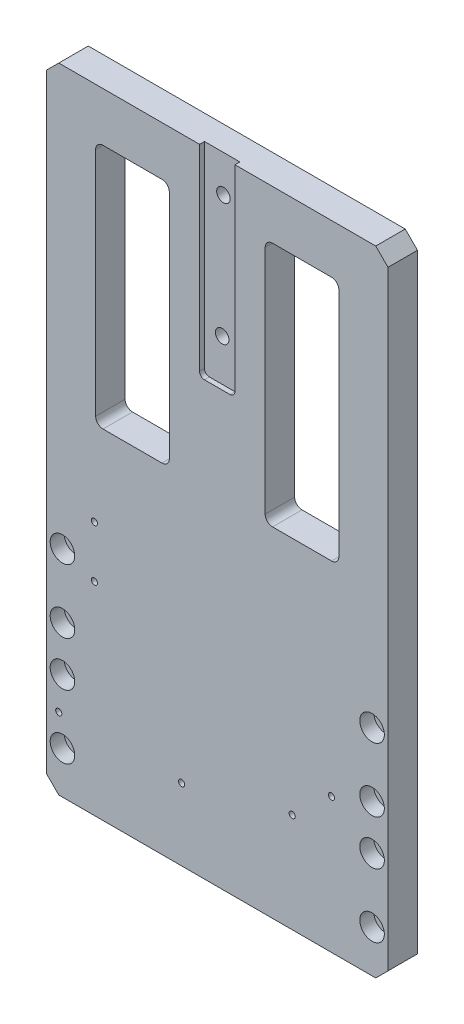
from build123d import *

# Parameters (mm, degrees)
SKETCH1_W                                            = 139
SKETCH1_H                                            = 258
BOSS_EXTRUDE1_DEPTH                                  = 12
CHAMFER1_SIZE                                        = 5
SKETCH2_W                                            = 30
SKETCH2_H                                            = 100
CUT_EXTRUDE1_DEPTH                                   = 237.506741929
SKETCH3_W                                            = 14.4
SKETCH3_H                                            = 82
CUT_EXTRUDE2_DEPTH                                   = 2
FILLET1_R                                            = 2
M3_TAPPED_HOLE1_D                                    = 2.5
M3_TAPPED_HOLE2_D                                    = 2.5
CBORE_FOR_M5_HEXAGON_SOCKET_HEAD_CAP_SCR_D           = 5.5
CBORE_FOR_M5_HEXAGON_SOCKET_HEAD_CAP_SCR_CBORE_D     = 10
CBORE_FOR_M5_HEXAGON_SOCKET_HEAD_CAP_SCR_CBORE_DEPTH = 5.7
FILLET2_R                                            = 3
CBORE_FOR_M5_HEXAGON_SOCKET_HEAD_CAP_2_D             = 5.5
CBORE_FOR_M5_HEXAGON_SOCKET_HEAD_CAP_2_DEPTH         = 11.5
CBORE_FOR_M5_HEXAGON_SOCKET_HEAD_CAP_2_CBORE_D       = 10
CBORE_FOR_M5_HEXAGON_SOCKET_HEAD_CAP_2_CBORE_DEPTH   = 5.7
CBORE_FOR_M5_HEXAGON_SOCKET_HEAD_CAP_2_TIP           = 1.652366702


with BuildPart() as part:
    # Sketch1 → Boss-Extrude1 (new body)
    with BuildSketch(Plane.XY):
        with Locations((50, 74.74294829)):
            Rectangle(SKETCH1_W, SKETCH1_H)
    extrude(amount=BOSS_EXTRUDE1_DEPTH)

    # Chamfer1
    chamfer1_edges = [part.edges().sort_by_distance(p)[0] for p in [
        (119.5, -54.25705171, 6),
        (-19.5, -54.25705171, 6),
        (-19.5, 203.74294829, 6),
        (119.5, 203.74294829, 6),
    ]]
    chamfer(chamfer1_edges, length=CHAMFER1_SIZE)

    # Sketch2 → Cut-Extrude1 (cut, through all)
    with BuildSketch(Plane.XY.offset(12)):
        with Locations((84.5, 133.74294829)):
            Rectangle(SKETCH2_W, SKETCH2_H)
        with Locations((15.5, 133.74294829)):
            Rectangle(SKETCH2_W, SKETCH2_H)
    extrude(amount=-CUT_EXTRUDE1_DEPTH, mode=Mode.SUBTRACT)

    # Sketch3 → Cut-Extrude2 (cut)
    with BuildSketch(Plane.XY.offset(12)):
        with Locations((50, 162.74294829)):
            Rectangle(SKETCH3_W, SKETCH3_H)
    extrude(amount=-CUT_EXTRUDE2_DEPTH, mode=Mode.SUBTRACT)

    # Fillet1
    fillet1_edges = [part.edges().sort_by_distance(p)[0] for p in [
        (57.2, 121.74294829, 11),
        (42.8, 121.74294829, 11),
    ]]
    fillet(fillet1_edges, radius=FILLET1_R)

    # M3 Tapped Hole1 (through all)
    with Locations(Plane.XY.offset(12)):
        with Locations((-14.5, -25.018399206), (35.5, -25.018399206), (96.5, 0.74294829), (80.5, -13.75705171)):
            Hole(M3_TAPPED_HOLE1_D / 2)

    # M3 Tapped Hole2 (through all)
    with Locations(Plane.XY.offset(12)):
        with Locations((0, 49.24294829), (0, 28.24294829)):
            Hole(M3_TAPPED_HOLE2_D / 2)

    # CBORE for M5 Hexagon socket head cap scr (through all)
    with Locations(Plane(origin=(0, 0, 0), x_dir=(-1, 0, 0), z_dir=(0, 0, -1))):
        with Locations((-50.5, 188.74294829), (-50, 138.745448352)):
            CounterBoreHole(CBORE_FOR_M5_HEXAGON_SOCKET_HEAD_CAP_SCR_D / 2, CBORE_FOR_M5_HEXAGON_SOCKET_HEAD_CAP_SCR_CBORE_D / 2, CBORE_FOR_M5_HEXAGON_SOCKET_HEAD_CAP_SCR_CBORE_DEPTH)

    # Fillet2
    fillet2_edges = [part.edges().sort_by_distance(p)[0] for p in [
        (99.5, 183.74294829, 6),
        (99.5, 83.74294829, 6),
        (69.5, 83.74294829, 6),
        (69.5, 183.74294829, 6),
        (30.5, 83.74294829, 6),
        (0.5, 83.74294829, 6),
        (0.5, 183.74294829, 6),
        (30.5, 183.74294829, 6),
    ]]
    fillet(fillet2_edges, radius=FILLET2_R)

    # CBORE for M5 Hexagon socket head cap 2
    with Locations(Plane.XY.offset(12)):
        with Locations((113, -37.05705171), (113, -11.05705171), (113, 7.24294829), (113, 33.24294829), (-13, -11.05705171), (-13, 7.2), (-13, -37.05705171), (-13, 33.24294829)):
            CounterBoreHole(CBORE_FOR_M5_HEXAGON_SOCKET_HEAD_CAP_2_D / 2, CBORE_FOR_M5_HEXAGON_SOCKET_HEAD_CAP_2_CBORE_D / 2, CBORE_FOR_M5_HEXAGON_SOCKET_HEAD_CAP_2_CBORE_DEPTH, depth=CBORE_FOR_M5_HEXAGON_SOCKET_HEAD_CAP_2_DEPTH)
            with Locations((0, 0, -(CBORE_FOR_M5_HEXAGON_SOCKET_HEAD_CAP_2_DEPTH + CBORE_FOR_M5_HEXAGON_SOCKET_HEAD_CAP_2_TIP / 2))):  # 118° drill point
                Cone(0, CBORE_FOR_M5_HEXAGON_SOCKET_HEAD_CAP_2_D / 2, CBORE_FOR_M5_HEXAGON_SOCKET_HEAD_CAP_2_TIP, mode=Mode.SUBTRACT)


solid = part.part
